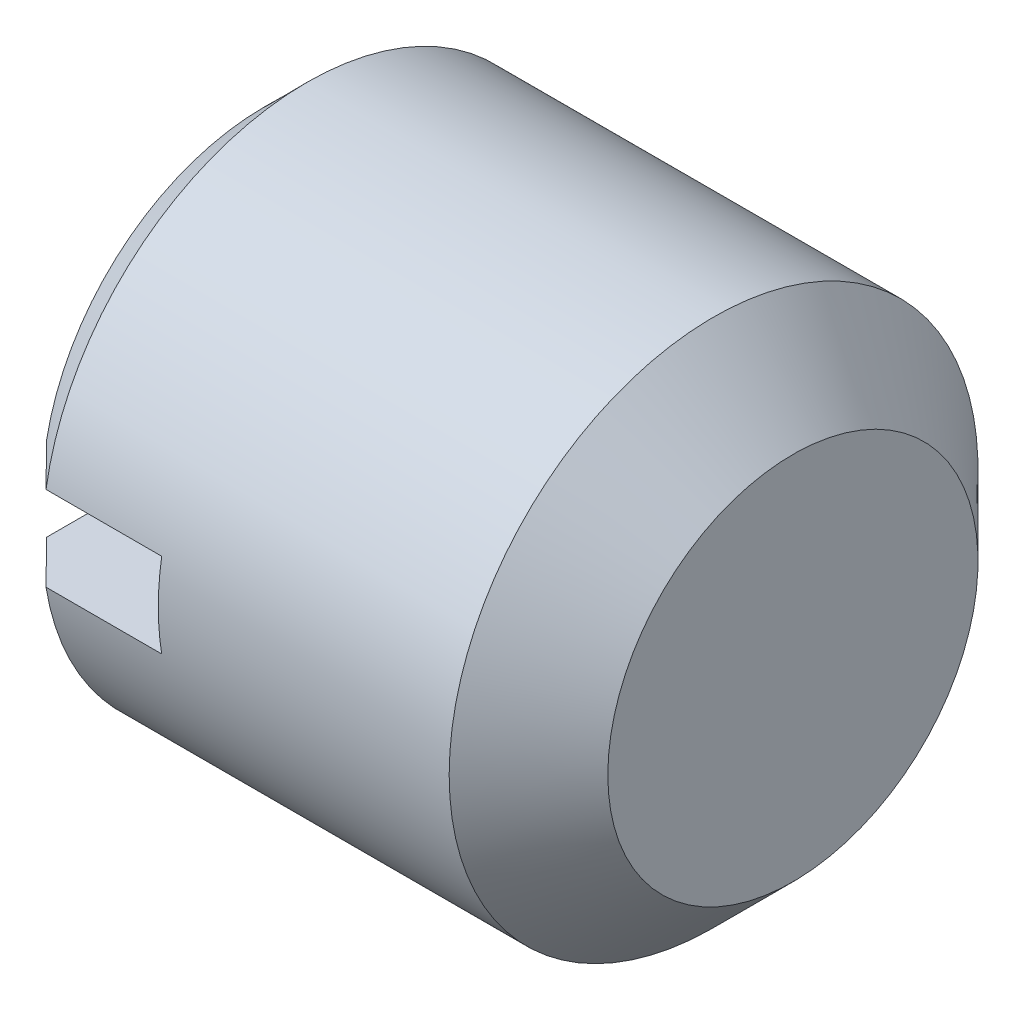
SolidWorks part; units mm, degrees
ref_plane "Front" through (0, 0, 0) normal (0, 0, 1) x (1, 0, 0)
ref_plane "Top" through (0, 0, 0) normal (0, 1, 0) x (1, 0, 0)
ref_plane "Right" through (0, 0, 0) normal (1, 0, 0) x (0, 0, -1)
sketch "Sketch1" plane through (0, 0, 0) normal (0, 0, 1) x (1, 0, 0)
  line L0 (0, 0) -> (10, 0)
  line L1 (10, 0) -> (10, 3.5)
  line L2 (10, 3.5) -> (8.5, 5)
  line L3 (8.5, 5) -> (0.812, 5)
  line L4 (0.812, 5) -> (0, 4.188)
  line L5 (0, 4.188) -> (0, 0)
  line L6 (-10.745, 0) -> (0.8952, 0) construction
revolve "Base" add sketch "Sketch1" angle 360 about L6
cosmetic thread "ThreadCosmetic1" [suppressed] parameters "D2"=8.376
sketch "Sketch2" plane through (0, 0, 0) normal (0, 0, 1) x (1, 0, 0)
  line L1 (0, 0.8) -> (3, 0.8)
  line L2 (0, 0.8) -> (0, -0.8)
  line L3 (0, -0.8) -> (3, -0.8)
  line L4 (3, 0.8) -> (3, -0.8)
  line L5 (0, 4.188) -> (0, -4.188) construction
extrude "Notch" cut sketch "Sketch2" against normal through all and the other way through all
sketch "Sketch3" plane through (0, 0, 0) normal (0, 0, 1) x (1, 0, 0)
  line L0 (0.812, 4.2968) -> (1.218, 5)
  line L1 (1.218, 5) -> (1.218, 5.812)
  line L2 (1.218, 5.812) -> (0.406, 5.812)
  line L3 (0.406, 5.812) -> (0.406, 5)
  line L4 (0.406, 5) -> (0.812, 4.2968)
  line L5 (0, 0) -> (1.5288, 0) construction
  line L6 (0.812, 5) -> (0.812, 0.8) construction
revolve "Cut-Revolve10" [suppressed] cut sketch "Sketch3" angle 360 about L5
pattern_linear "LPattern10" [suppressed] count 9 spacing 0.9744 along (1, 0, 0)
equation "\"df@Sketch1\" = \"D2@ThreadCosmetic1\""
equation "\"m@Sketch2\" = \"n@Sketch2\" / 2"
equation "\"D1@Sketch3\" = \"d@Sketch1\""
equation "\"D2@Sketch3\" =  ( \"d@Sketch1\" - \"D2@ThreadCosmetic1\" )  / 2"
equation "\"D3@LPattern10\" = \"D2@Sketch3\" * 1.2"
equation "\"D1@LPattern10\" =  ( \"l@Sketch1\" -  ( \"d@Sketch1\" - \"df@Sketch1\" )  / 2 )  / \"D3@LPattern10\""
